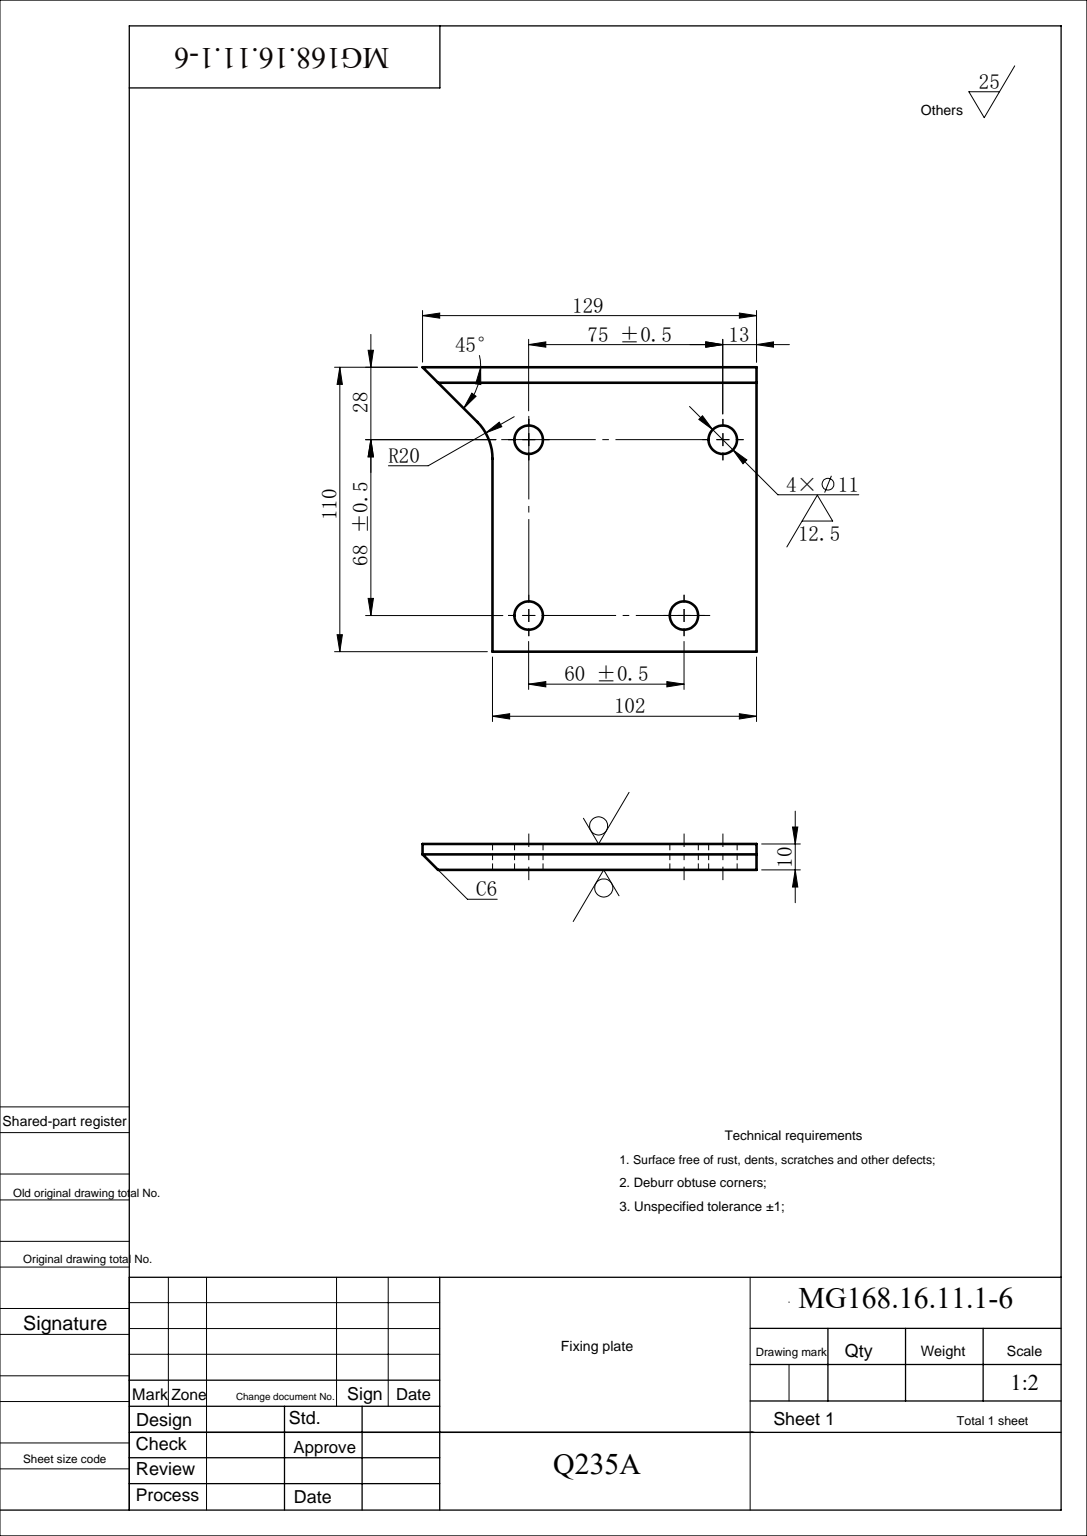
from build123d import *

# Parameters (mm, degrees)
BOSS_EXTRUDE1_DEPTH     = 5
CUT_EXTRUDE1_DEPTH      = 120.507321951
CUT_EXTRUDE1_DEPTH_BACK = 120.507321951
SKETCH2_R               = 5.5
CHAMFER1_SIZE           = 6


with BuildPart() as part:
    # Sketch1 → Boss-Extrude1 (new, symmetric)
    with BuildSketch(Plane.XY):
        with BuildLine():
            Line((-58, 96), (71, 96))
            Line((71, 96), (49.857864376, 74.857864376))
            ThreePointArc((49.857864376, 74.857864376), (45.52240935, 68.3693974), (44, 60.715728753))
            Line((44, 60.715728753), (44, -14))
            Line((44, -14), (-58, -14))
            Line((-58, -14), (-58, 96))
        make_face()
    extrude(amount=BOSS_EXTRUDE1_DEPTH, both=True)

    # Sketch2 → Cut-Extrude1 (cut, two sides: drawn at the far end of the back side and taken through both)
    with BuildSketch(Plane.XY.offset(-CUT_EXTRUDE1_DEPTH_BACK)):
        with Locations((-30, 0)):
            Circle(SKETCH2_R)
        with Locations((30, 0)):
            Circle(SKETCH2_R)
        with Locations((-45, 68)):
            Circle(SKETCH2_R)
        with Locations((30, 68)):
            Circle(SKETCH2_R)
    extrude(amount=CUT_EXTRUDE1_DEPTH + CUT_EXTRUDE1_DEPTH_BACK, mode=Mode.SUBTRACT)

    # Chamfer1
    chamfer1_edges = [part.edges().sort_by_distance(p)[0] for p in [
        (6.5, 96, -5),
    ]]
    chamfer(chamfer1_edges, length=CHAMFER1_SIZE)


solid = part.part
